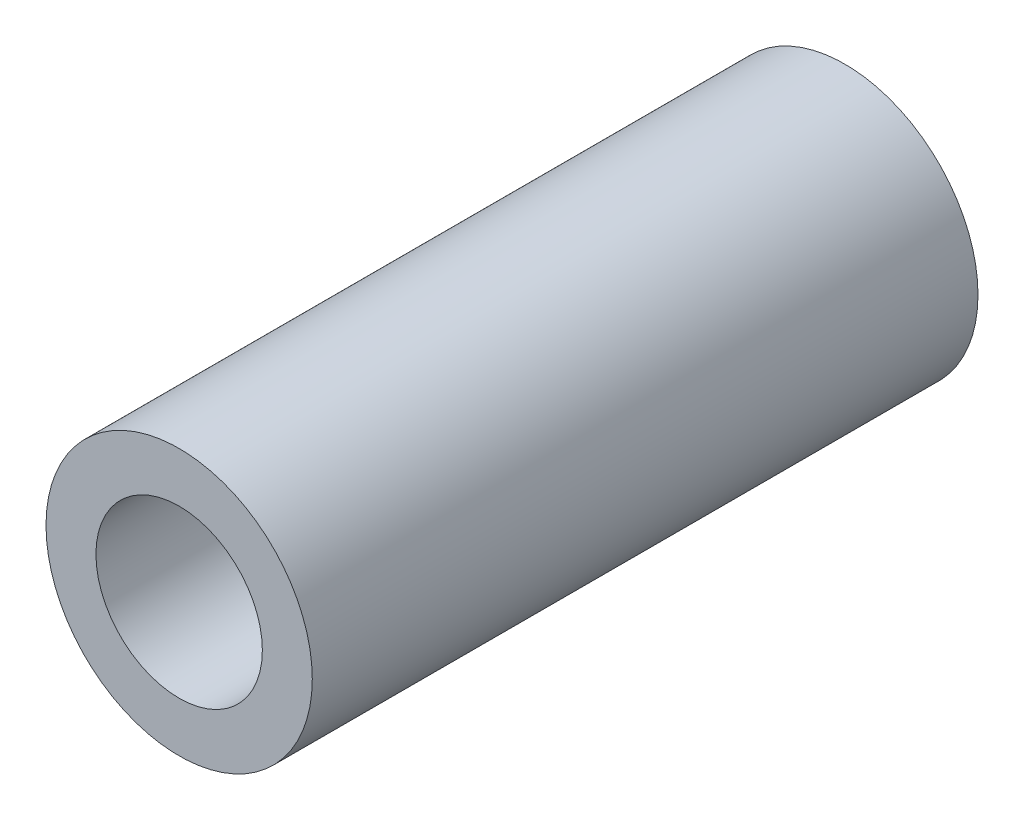
SolidWorks part; units mm, degrees
material "AISI 1015 steel, cold drawn (SS)"
ref_plane "Front Plane" through (0, 0, 0) normal (0, 0, 1) x (1, 0, 0)
ref_plane "Top Plane" through (0, 0, 0) normal (0, 1, 0) x (1, 0, 0)
ref_plane "Right Plane" through (0, 0, 0) normal (1, 0, 0) x (0, 0, -1)
sketch "Sketch1" plane through (0, 0, 0) normal (0, 0, 1) x (1, 0, 0)
  circle A0 centre (0, 0) radius 8
extrude "Boss-Extrude1" add sketch "Sketch1" along normal blind 40
sketch "Sketch2" plane through (0, 0, 40) normal (0, 0, 1) x (1, 0, 0)
  circle A0 centre (0, 0) radius 5
extrude "Cut-Extrude1" cut sketch "Sketch2" against normal blind 33
